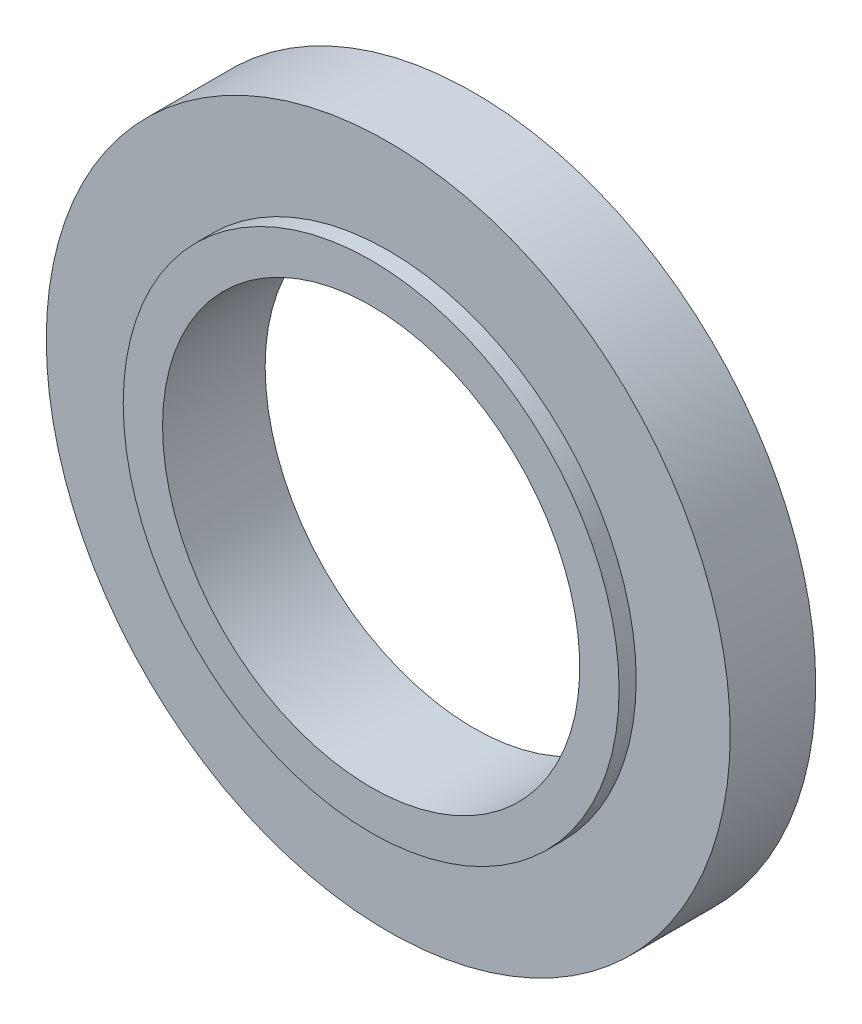
from build123d import *


with BuildPart() as part:
    # Sketch1 → Revolve1 (revolve)
    with BuildSketch(Plane.XZ, mode=Mode.PRIVATE) as revolve1_sk:
        Polygon((6.1, 1.5), (6.1, -1.5), (10, -1.5), (10, 1), (7.25, 1), (7.25, 1.5), align=None)
    revolve(revolve1_sk.sketch.rotate(Axis((0, 0, 1.5), (0, 0, -1)), 180), axis=Axis((0, 0, 1.5), (0, 0, -1)))


solid = part.part
